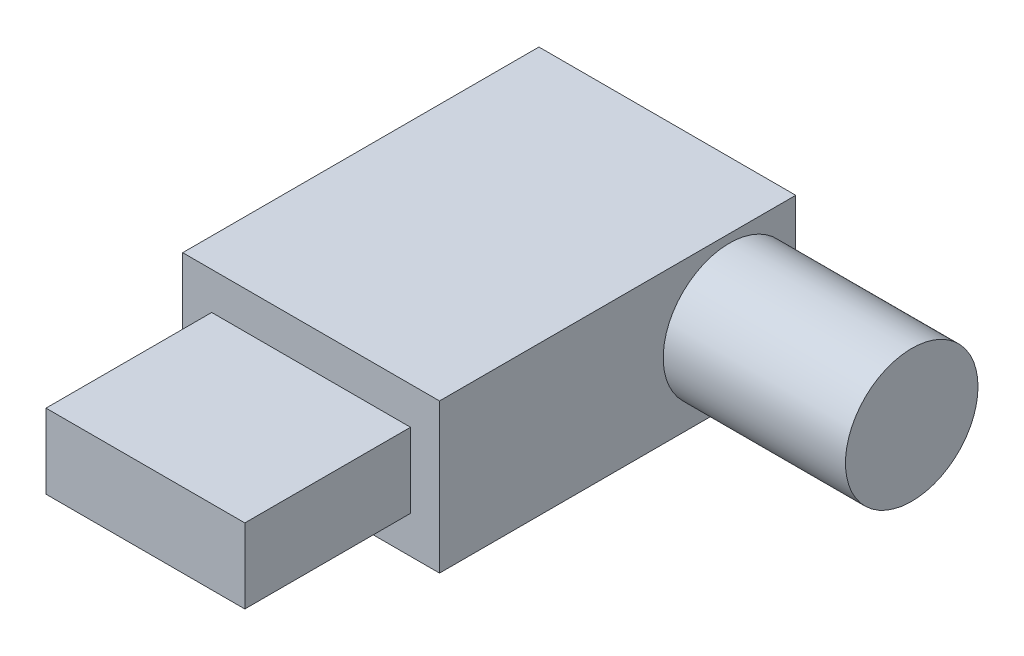
from build123d import *

# Parameters (mm, degrees)
SKETCH_1_W      = 15.5
SKETCH_1_H      = 9
EXTRUDE_1_DEPTH = 21.5
SKETCH_2_R      = 4
EXTRUDE_2_DEPTH = 11
SKETCH_3_W      = 12
SKETCH_3_H      = 4.5
EXTRUDE_3_DEPTH = 10


with BuildPart() as part:
    # 草图1 → 凸台-拉伸1 (new body)
    with BuildSketch(Plane.XY):
        Rectangle(SKETCH_1_W, SKETCH_1_H)
    extrude(amount=-EXTRUDE_1_DEPTH)

    # 草图2 → 凸台-拉伸2 (add)
    with BuildSketch(Plane(origin=(7.75, 0, 0), x_dir=(0, 0, -1), z_dir=(1, 0, 0))):
        with Locations((17.5, 0)):
            Circle(SKETCH_2_R)
    extrude(amount=EXTRUDE_2_DEPTH)

    # 草图3 → 凸台-拉伸3 (add)
    with BuildSketch(Plane.XY):
        Rectangle(SKETCH_3_W, SKETCH_3_H)
    extrude(amount=EXTRUDE_3_DEPTH)


solid = part.part
